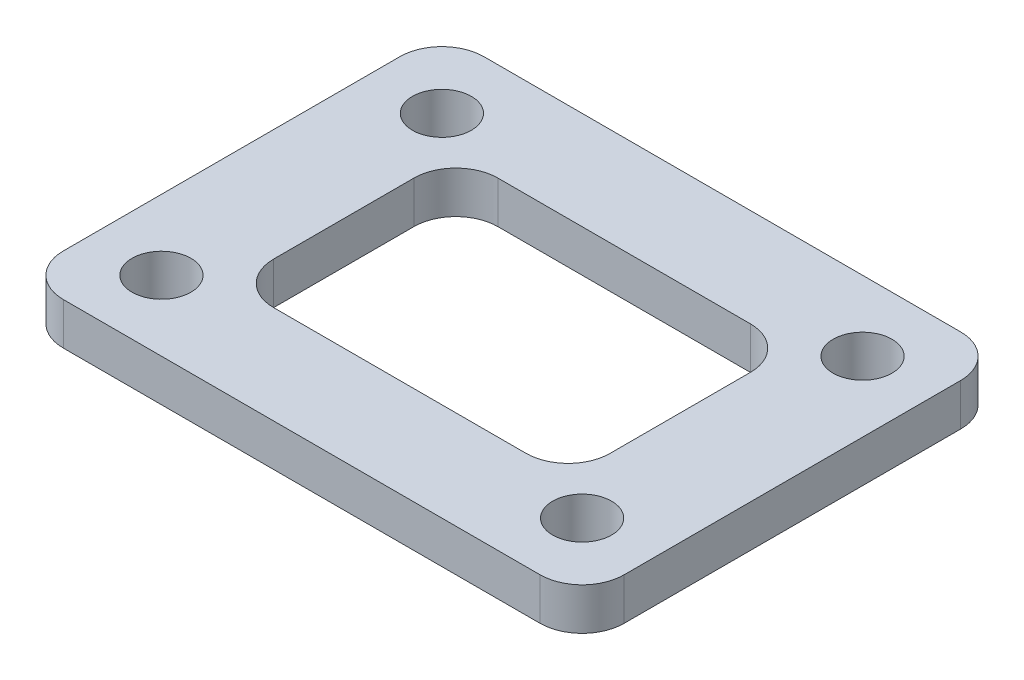
SolidWorks part; units mm, degrees
material "哈碳纤"
ref_plane "前视基准面" through (0, 0, 0) normal (0, 0, 1) x (1, 0, 0)
ref_plane "上视基准面" through (0, 0, 0) normal (0, 1, 0) x (1, 0, 0)
ref_plane "右视基准面" through (0, 0, 0) normal (1, 0, 0) x (0, 0, -1)
other "Configuration Table"
sketch "草图1" plane through (0, 0, 0) normal (0, 1, 0) x (1, 0, 0)
  line L1 (-17, -15) -> (17, -15)
  line L2 (-20, -12) -> (-20, 12)
  line L3 (-17, 15) -> (17, 15)
  line L4 (20, -12) -> (20, 12)
  line L5 (-20, -15) -> (20, 15) construction
  line L6 (-20, 15) -> (20, -15) construction
  line L7 (-15, -10) -> (15, -10) construction
  line L8 (-15, -10) -> (-15, 10) construction
  line L9 (-15, 10) -> (15, 10) construction
  line L10 (15, -10) -> (15, 10) construction
  line L11 (-15, -10) -> (15, 10) construction
  line L12 (-15, 10) -> (15, -10) construction
  line L13 (-9, -8) -> (9, -8)
  line L14 (-12, -5) -> (-12, 5)
  line L15 (-9, 8) -> (9, 8)
  line L16 (12, -5) -> (12, 5)
  line L17 (-12, -8) -> (12, 8) construction
  line L18 (-12, 8) -> (12, -8) construction
  circle A0 centre (-15, 10) radius 2.1
  circle A1 centre (15, 10) radius 2.1
  circle A2 centre (-15, -10) radius 2.1
  circle A3 centre (15, -10) radius 2.1
  arc A4 (17, -15) -> (20, -12) centre (17, -12) ccw
  arc A5 (-20, 12) -> (-17, 15) centre (-17, 12) cw
  arc A6 (-17, -15) -> (-20, -12) centre (-17, -12) cw
  arc A7 (17, 15) -> (20, 12) centre (17, 12) cw
  arc A8 (9, -8) -> (12, -5) centre (9, -5) ccw
  arc A9 (-12, 5) -> (-9, 8) centre (-9, 5) cw
  arc A10 (-9, -8) -> (-12, -5) centre (-9, -5) cw
  arc A11 (9, 8) -> (12, 5) centre (9, 5) cw
  point P0 (0, 0)
  point P5 (0, 0)
  point P27 (0, 0)
  dimension "D5" = 4.2
  dimension "D6" = 3
  dimension "D9" = 3
  dimension "D1" = 30
  dimension "D2" = 40
  dimension "D3" = 20
  dimension "D4" = 30
  dimension "D7" = 16
  dimension "D8" = 24
extrude "凸台-拉伸1" add sketch "草图1" along normal blind 3
